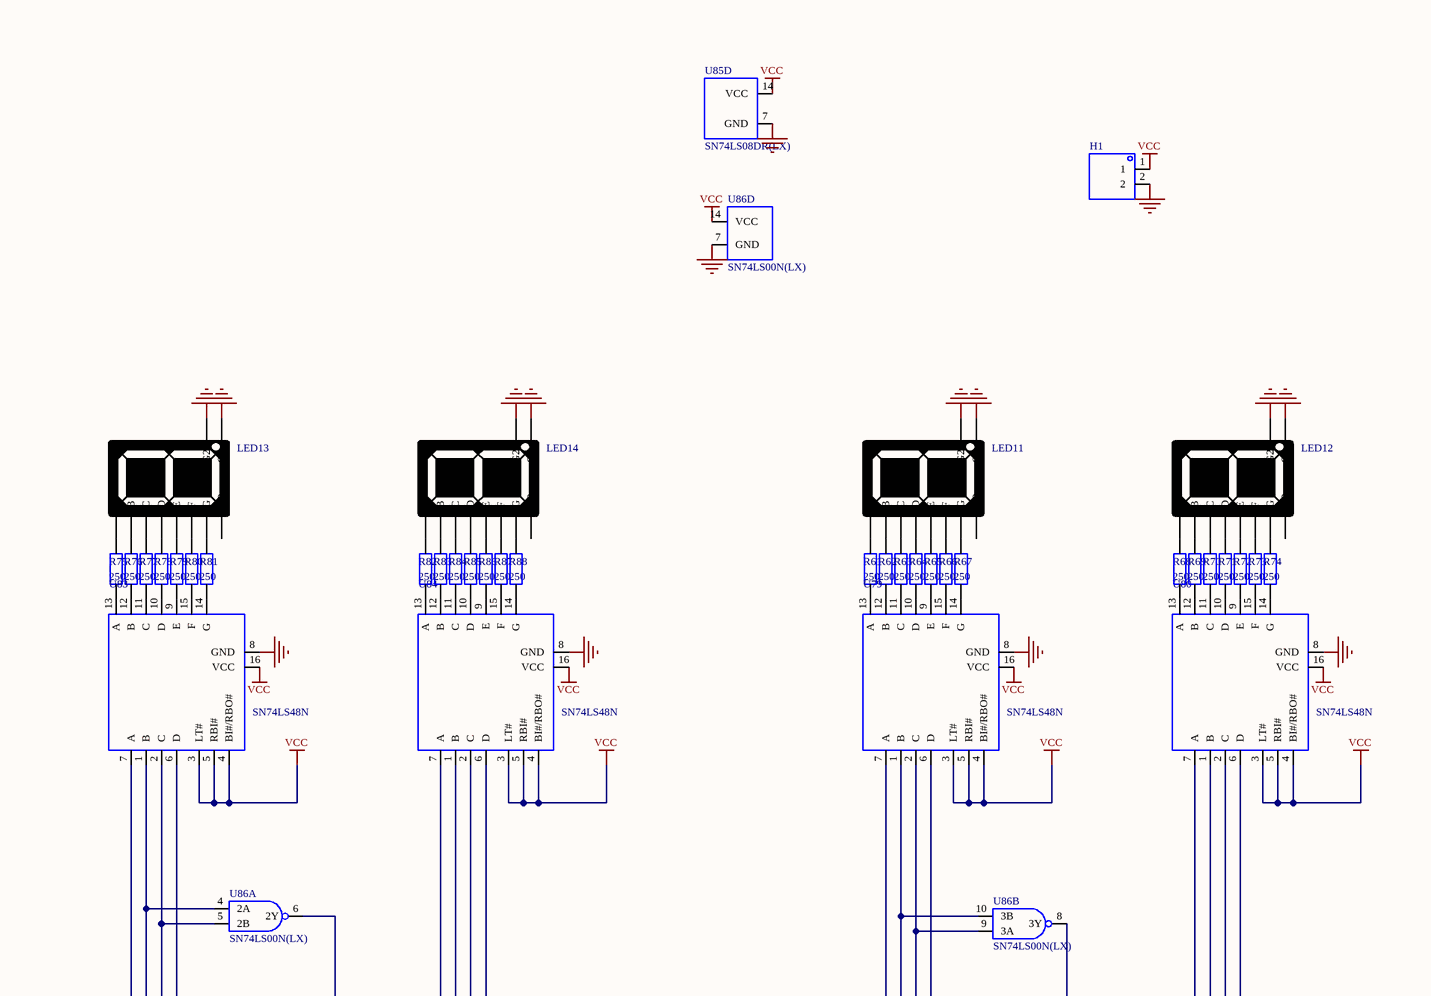
[diagram p0: MISC52151-3.schdoc, top left]
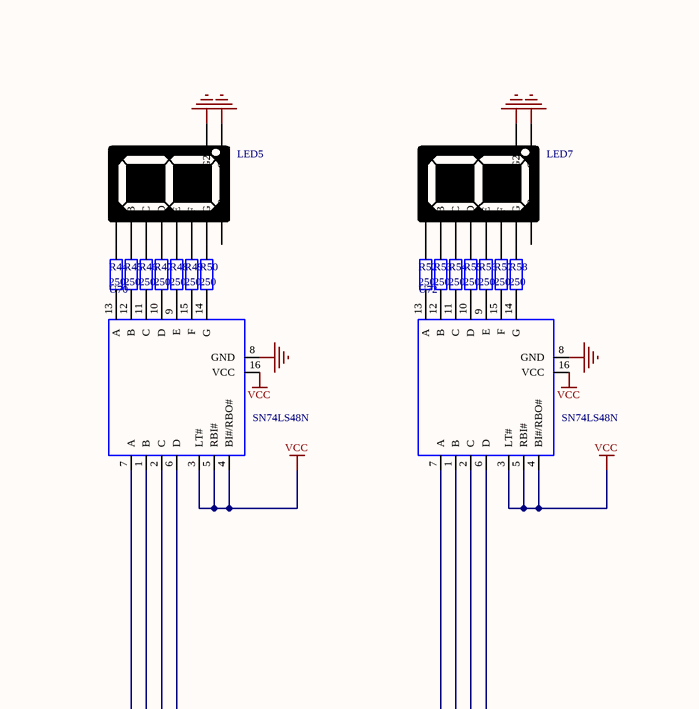
[diagram p1: MISC52151-3.schdoc, top right]
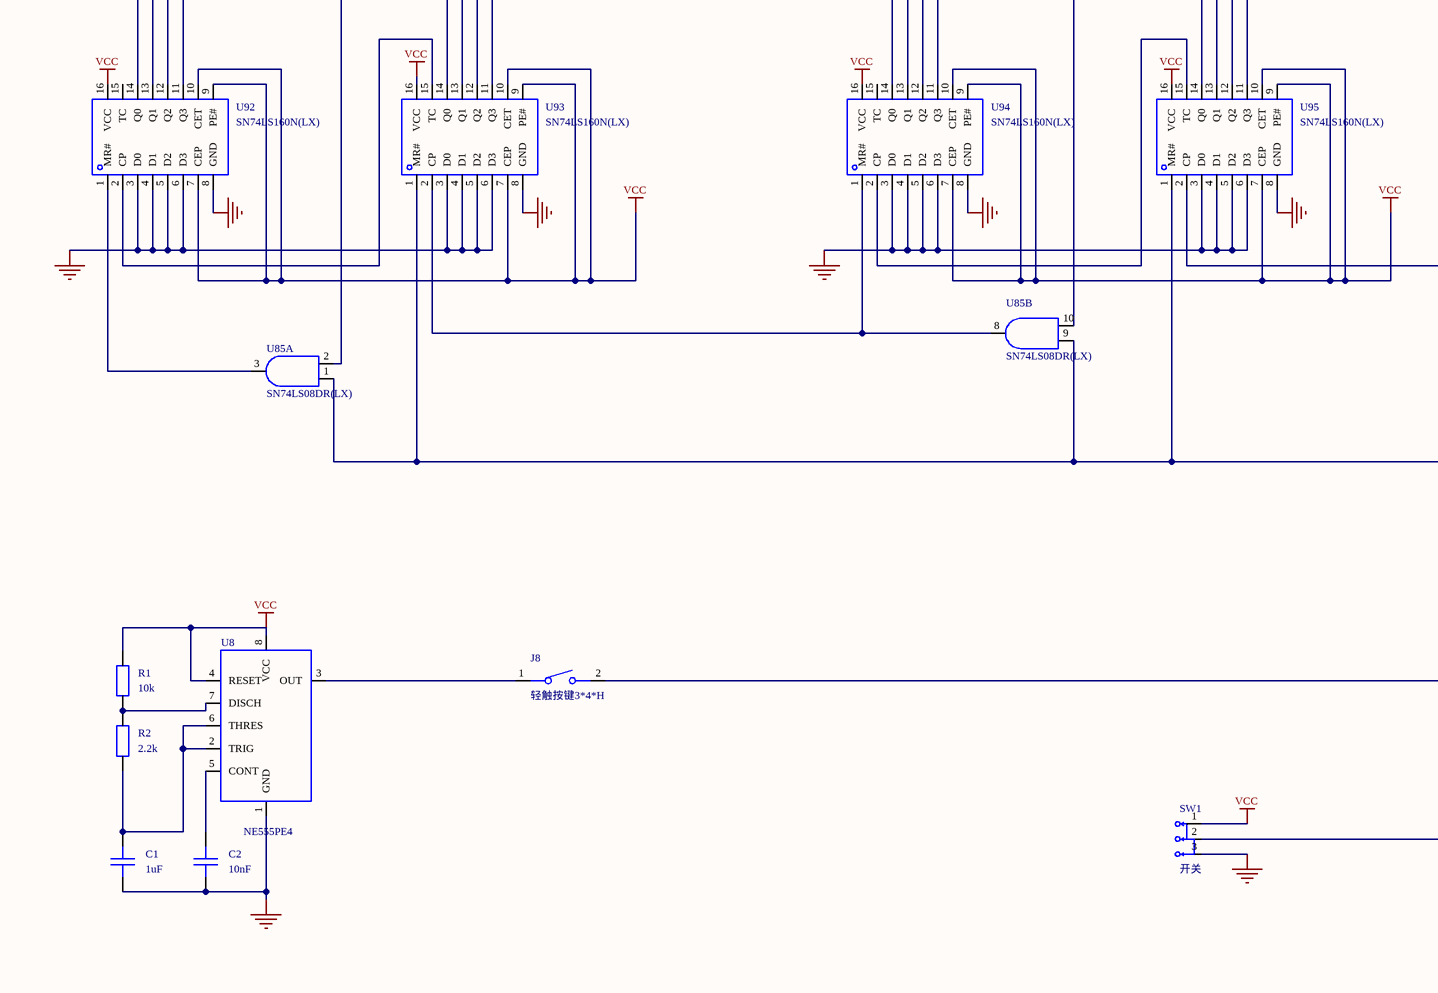
[diagram p2: MISC52151-3.schdoc, bottom left]
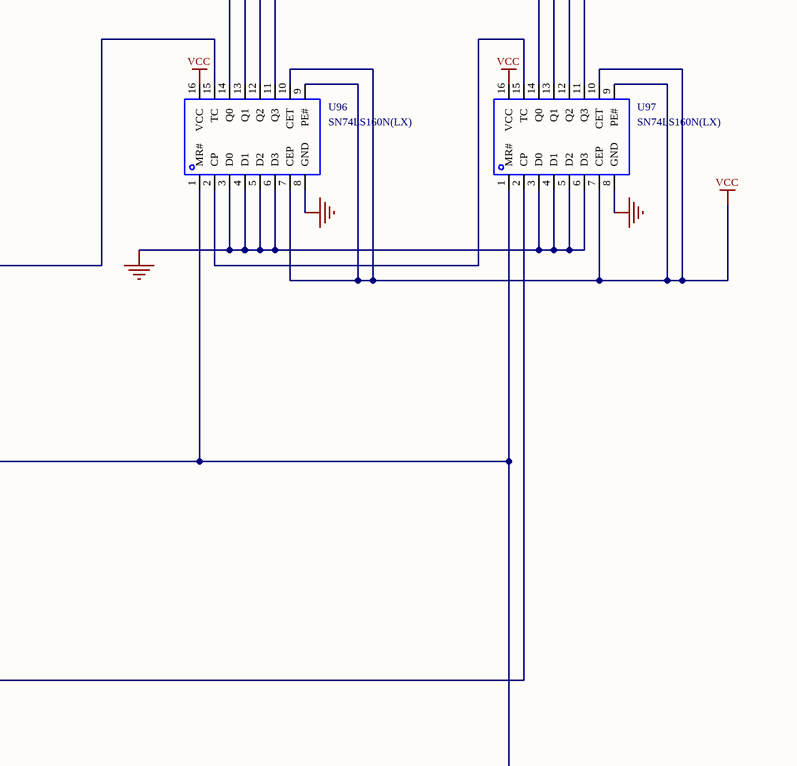
[diagram p3: MISC52151-3.schdoc, bottom right]
# Altium project MISC52151-2.PrjPcb
1 sheet, 70 parts. Net scope: global (net labels, ports and power ports of the same name join across sheets).
Board file: MISC52151.pcbdoc

## Sheet MISC52151-3.schdoc
size 178 x 98 mm; Version: V1.0; @Project Name: MISC52151; @Page Count: 1; @Update Date: 2025-06-06; @Create Date: 2025-06-06; @Schematic Name: MISC52151; @Page No: 1; @Board Name: MISC52151; @Create Time: 20:33:48; @Update Time: 02:46:09

### Parts
C1  1uF  [C0805]
C2  10nF  [C0805]
H1  (no value)  [HDR-TH_2P-P2.54-V-M-1]
J8  轻触按键3*4*H  [SW-SMD_L4.0-W2.9-LS5.0]
LED5  (no value)  [LED-SEG-TH_10P-L12.6-W19.0-P2.54-S15.24-BL]
LED7  (no value)  [LED-SEG-TH_10P-L12.6-W19.0-P2.54-S15.24-BL]
LED11  (no value)  [LED-SEG-TH_10P-L12.6-W19.0-P2.54-S15.24-BL]
LED12  (no value)  [LED-SEG-TH_10P-L12.6-W19.0-P2.54-S15.24-BL]
LED13  (no value)  [LED-SEG-TH_10P-L12.6-W19.0-P2.54-S15.24-BL]
LED14  (no value)  [LED-SEG-TH_10P-L12.6-W19.0-P2.54-S15.24-BL]
R1  10k  [R0603]
R2  2.2k  [R0603]
R44  250  [R0603]
R45  250  [R0603]
R46  250  [R0603]
R47  250  [R0603]
R48  250  [R0603]
R49  250  [R0603]
R50  250  [R0603]
R52  250  [R0603]
R53  250  [R0603]
R54  250  [R0603]
R55  250  [R0603]
R56  250  [R0603]
R57  250  [R0603]
R58  250  [R0603]
R61  250  [R0603]
R62  250  [R0603]
R63  250  [R0603]
R64  250  [R0603]
R65  250  [R0603]
R66  250  [R0603]
R67  250  [R0603]
R68  250  [R0603]
R69  250  [R0603]
R70  250  [R0603]
R71  250  [R0603]
R72  250  [R0603]
R73  250  [R0603]
R74  250  [R0603]
R75  250  [R0603]
R76  250  [R0603]
R77  250  [R0603]
R78  250  [R0603]
R79  250  [R0603]
R80  250  [R0603]
R81  250  [R0603]
R82  250  [R0603]
R83  250  [R0603]
R84  250  [R0603]
R85  250  [R0603]
R86  250  [R0603]
R87  250  [R0603]
R88  250  [R0603]
SW1  开关  [SW-TH_SS-12D01-GX]
U8  NE555PE4  [PDIP-8_L9.6-W6.4-P2.54-LS7.9-BL-1]
U70  SN74LS48N  [DIP-16_L19.3-W6.4-P2.54-LS7.6-BL]
U72  SN74LS48N  [DIP-16_L19.3-W6.4-P2.54-LS7.6-BL]
U79  SN74LS48N  [DIP-16_L19.3-W6.4-P2.54-LS7.6-BL]
U80  SN74LS48N  [DIP-16_L19.3-W6.4-P2.54-LS7.6-BL]
U83  SN74LS48N  [DIP-16_L19.3-W6.4-P2.54-LS7.6-BL]
U84  SN74LS48N  [DIP-16_L19.3-W6.4-P2.54-LS7.6-BL]
U85  SN74LS08DR(LX)  [SOIC-14_L8.7-W3.9-P1.27-LS6.0-BL]  (parts A,B,D of 4)
U86  SN74LS00N(LX)  [PDIP-14_L19.3-W6.4-P2.54-LS7.9-BL]  (parts A,B,D of 4)
U92  SN74LS160N(LX)  [DIP-16_L19.4-W6.4-P2.54-S7.6-BL]
U93  SN74LS160N(LX)  [DIP-16_L19.4-W6.4-P2.54-S7.6-BL]
U94  SN74LS160N(LX)  [DIP-16_L19.4-W6.4-P2.54-S7.6-BL]
U95  SN74LS160N(LX)  [DIP-16_L19.4-W6.4-P2.54-S7.6-BL]
U96  SN74LS160N(LX)  [DIP-16_L19.4-W6.4-P2.54-S7.6-BL]
U97  SN74LS160N(LX)  [DIP-16_L19.4-W6.4-P2.54-S7.6-BL]

### Nets
GND: C1.1 C2.1 H1.2 LED5.3(G1) LED5.8(G2) LED7.3(G1) LED7.8(G2) LED11.3(G1) LED11.8(G2) LED12.3(G1) LED12.8(G2) LED13.3(G1) LED13.8(G2) LED14.3(G1) LED14.8(G2) SW1.3 U8.1(GND) U70.8(GND) U72.8(GND) U79.8(GND) U80.8(GND) U83.8(GND) U84.8(GND) U85.7(GND) U86.7(GND) U92.3(D0) U92.4(D1) U92.5(D2) U92.6(D3) U92.8(GND) U93.3(D0) U93.4(D1) U93.5(D2) U93.6(D3) U93.8(GND) U94.3(D0) U94.4(D1) U94.5(D2) U94.6(D3) U94.8(GND) U95.3(D0) U95.4(D1) U95.5(D2) U95.6(D3) U95.8(GND) U96.3(D0) U96.4(D1) U96.5(D2) U96.6(D3) U96.8(GND) U97.3(D0) U97.4(D1) U97.5(D2) U97.6(D3) U97.8(GND)
VCC: H1.1 R1.2 SW1.1 U8.4(RESET) U8.8(VCC) U70.3(LT#) U70.4(BI#/RBO#) U70.5(RBI#) U70.16(VCC) U72.3(LT#) U72.4(BI#/RBO#) U72.5(RBI#) U72.16(VCC) U79.3(LT#) U79.4(BI#/RBO#) U79.5(RBI#) U79.16(VCC) U80.3(LT#) U80.4(BI#/RBO#) U80.5(RBI#) U80.16(VCC) U83.3(LT#) U83.4(BI#/RBO#) U83.5(RBI#) U83.16(VCC) U84.3(LT#) U84.4(BI#/RBO#) U84.5(RBI#) U84.16(VCC) U85.14(VCC) U86.14(VCC) U92.7(CEP) U92.9(PE#) U92.10(CET) U92.16(VCC) U93.7(CEP) U93.9(PE#) U93.10(CET) U93.16(VCC) U94.7(CEP) U94.9(PE#) U94.10(CET) U94.16(VCC) U95.7(CEP) U95.9(PE#) U95.10(CET) U95.16(VCC) U96.7(CEP) U96.9(PE#) U96.10(CET) U96.16(VCC) U97.7(CEP) U97.9(PE#) U97.10(CET) U97.16(VCC)
NetC1_2: C1.2 R2.1 U8.2(TRIG) U8.6(THRES)
NetC2_2: C2.2 U8.5(CONT)
NetJ8_1: J8.1 U8.3(OUT)
NetJ8_2: J8.2 U97.2(CP)
NetLED5_1: LED5.1(E) R48.2
NetLED5_2: LED5.2(D) R47.2
NetLED5_4: LED5.4(C) R46.2
NetLED5_6: LED5.6(B) R45.2
NetLED5_7: LED5.7(A) R44.2
NetLED5_9: LED5.9(F) R49.2
NetLED5_10: LED5.10(G) R50.2
NetLED7_1: LED7.1(E) R56.2
NetLED7_2: LED7.2(D) R55.2
NetLED7_4: LED7.4(C) R54.2
NetLED7_6: LED7.6(B) R53.2
NetLED7_7: LED7.7(A) R52.2
NetLED7_9: LED7.9(F) R57.2
NetLED7_10: LED7.10(G) R58.2
NetLED11_1: LED11.1(E) R65.2
NetLED11_2: LED11.2(D) R64.2
NetLED11_4: LED11.4(C) R63.2
NetLED11_6: LED11.6(B) R62.2
NetLED11_7: LED11.7(A) R61.2
NetLED11_9: LED11.9(F) R66.2
NetLED11_10: LED11.10(G) R67.2
NetLED12_1: LED12.1(E) R72.2
NetLED12_2: LED12.2(D) R71.2
NetLED12_4: LED12.4(C) R70.2
NetLED12_6: LED12.6(B) R69.2
NetLED12_7: LED12.7(A) R68.2
NetLED12_9: LED12.9(F) R73.2
NetLED12_10: LED12.10(G) R74.2
NetLED13_1: LED13.1(E) R79.2
NetLED13_2: LED13.2(D) R78.2
NetLED13_4: LED13.4(C) R77.2
NetLED13_6: LED13.6(B) R76.2
NetLED13_7: LED13.7(A) R75.2
NetLED13_9: LED13.9(F) R80.2
NetLED13_10: LED13.10(G) R81.2
NetLED14_1: LED14.1(E) R86.2
NetLED14_2: LED14.2(D) R85.2
NetLED14_4: LED14.4(C) R84.2
NetLED14_6: LED14.6(B) R83.2
NetLED14_7: LED14.7(A) R82.2
NetLED14_9: LED14.9(F) R87.2
NetLED14_10: LED14.10(G) R88.2
NetR1_1: R1.1 R2.2 U8.7(DISCH)
NetR44_1: R44.1 U70.13(A)
NetR45_1: R45.1 U70.12(B)
NetR46_1: R46.1 U70.11(C)
NetR47_1: R47.1 U70.10(D)
NetR48_1: R48.1 U70.9(E)
NetR49_1: R49.1 U70.15(F)
NetR50_1: R50.1 U70.14(G)
NetR52_1: R52.1 U72.13(A)
NetR53_1: R53.1 U72.12(B)
NetR54_1: R54.1 U72.11(C)
NetR55_1: R55.1 U72.10(D)
NetR56_1: R56.1 U72.9(E)
NetR57_1: R57.1 U72.15(F)
NetR58_1: R58.1 U72.14(G)
NetR61_1: R61.1 U79.13(A)
NetR62_1: R62.1 U79.12(B)
NetR63_1: R63.1 U79.11(C)
NetR64_1: R64.1 U79.10(D)
NetR65_1: R65.1 U79.9(E)
NetR66_1: R66.1 U79.15(F)
NetR67_1: R67.1 U79.14(G)
NetR68_1: R68.1 U80.13(A)
NetR69_1: R69.1 U80.12(B)
NetR70_1: R70.1 U80.11(C)
NetR71_1: R71.1 U80.10(D)
NetR72_1: R72.1 U80.9(E)
NetR73_1: R73.1 U80.15(F)
NetR74_1: R74.1 U80.14(G)
NetR75_1: R75.1 U83.13(A)
NetR76_1: R76.1 U83.12(B)
NetR77_1: R77.1 U83.11(C)
NetR78_1: R78.1 U83.10(D)
NetR79_1: R79.1 U83.9(E)
NetR80_1: R80.1 U83.15(F)
NetR81_1: R81.1 U83.14(G)
NetR82_1: R82.1 U84.13(A)
NetR83_1: R83.1 U84.12(B)
NetR84_1: R84.1 U84.11(C)
NetR85_1: R85.1 U84.10(D)
NetR86_1: R86.1 U84.9(E)
NetR87_1: R87.1 U84.15(F)
NetR88_1: R88.1 U84.14(G)
NetSW1_2: SW1.2 U85.1(1A) U85.9(3A) U93.1(MR#) U95.1(MR#) U96.1(MR#) U97.1(MR#)
NetU70_1: U70.1(B) U96.13(Q1)
NetU70_2: U70.2(C) U96.12(Q2)
NetU70_6: U70.6(D) U96.11(Q3)
NetU70_7: U70.7(A) U96.14(Q0)
NetU72_1: U72.1(B) U97.13(Q1)
NetU72_2: U72.2(C) U97.12(Q2)
NetU72_6: U72.6(D) U97.11(Q3)
NetU72_7: U72.7(A) U97.14(Q0)
NetU79_1: U79.1(B) U86.10(3B) U94.13(Q1)
NetU79_2: U79.2(C) U86.9(3A) U94.12(Q2)
NetU79_6: U79.6(D) U94.11(Q3)
NetU79_7: U79.7(A) U94.14(Q0)
NetU80_1: U80.1(B) U95.13(Q1)
NetU80_2: U80.2(C) U95.12(Q2)
NetU80_6: U80.6(D) U95.11(Q3)
NetU80_7: U80.7(A) U95.14(Q0)
NetU83_1: U83.1(B) U86.4(2A) U92.13(Q1)
NetU83_2: U83.2(C) U86.5(2B) U92.12(Q2)
NetU83_6: U83.6(D) U92.11(Q3)
NetU83_7: U83.7(A) U92.14(Q0)
NetU84_1: U84.1(B) U93.13(Q1)
NetU84_2: U84.2(C) U93.12(Q2)
NetU84_6: U84.6(D) U93.11(Q3)
NetU84_7: U84.7(A) U93.14(Q0)
NetU85_2: U85.2(1B) U86.6(2Y)
NetU85_3: U85.3(1Y) U92.1(MR#)
NetU85_8: U85.8(3Y) U93.2(CP) U94.1(MR#)
NetU85_10: U85.10(3B) U86.8(3Y)
NetU92_2: U92.2(CP) U93.15(TC)
NetU94_2: U94.2(CP) U95.15(TC)
NetU95_2: U95.2(CP) U96.15(TC)
NetU96_2: U96.2(CP) U97.15(TC)

Not connected (* = marked no-connect by the designer): LED5 5(DP); LED7 5(DP); LED11 5(DP); LED12 5(DP); LED13 5(DP); LED14 5(DP); U92 15(TC); U94 15(TC)

### Notes on the sheet
- 2025-06-06
- 原理图
- P1
- 版本
- 尺寸
- 页
- 共
- A4
- 1

### Library data of the parts
C1 C2 = CAP_0805: ConvertToPcb: yes; SymbolName: CapAcitance; ModelId: 1ba041120af144c991958decab20d241; ModelName: C0805_L2.0-W1.3-H1.3; ModelTransform: 78.74,51.181,0,0,0,0,0,0.0005,0; Device: CAP_0805; AddInBom: yes; Supplier Footprint: 0805; FootprintName: C0805
  C1: Value: 1uF
  C2: Value: 10nF
H1 = HDR-M_2.54_1x2P: Symbol: 210S-1*2P L=11.6MMGold-plated black; ConvertToPcb: yes; ModelId: 79b2e9f2d70a4d68a1b7098f27c6d4c5; ModelName: HDR-M-2.54_1x2; ModelTransform: 200,100,0,0,0,0,0,0,-118.11; Device: HDR-M_2.54_1x2P; AddInBom: yes; SupplierPart: C124375; Supplier Footprint: 插件; FootprintName: HDR-TH_2P-P2.54-V-M-1
J8 = 轻触按键3*4*H: AddInBom: yes; ModelId: 63599cce708d48afbce1b0db00354477; ModelName: SW-SMD_L4.0-W2.9-H2-LS5.0; ModelTransform: 196.85,114.173,0,0,0,0,0,0,0; Symbol: 轻触按键3*4*H; Device: 轻触按键3*4*H; LCSC Part Name: 轻触按键3*4*H; SupplierPart: C9900017573; ManufacturerPart: 轻触按键3*4*H; Supplier Footprint: 轻触按键3*4*2.5; Supplier: LCSC; ConvertToPcb: yes; FootprintName: SW-SMD_L4.0-W2.9-LS5.0
LED5 LED7 LED11-LED14 = LED_SEG_TH_0.56x1: Symbol: LED_SEG_TH_0.56*1; ConvertToPcb: yes; ModelId: 16c3aae6d39e4ecc9e744d6eeac8d57b; ModelName: LED-SEG-TH_0.56_1p; ModelTransform: 496.062,748.03,0,0,0,0,0,0,-137.795; Device: LED_SEG_TH_0.56x1; AddInBom: yes; Supplier Footprint: 插件; FootprintName: LED-SEG-TH_10P-L12.6-W19.0-P2.54-S15.24-BL
R1 R2 R44-R50 R52-R58 R61-R88 = Res_0603: Symbol: 电阻; ConvertToPcb: yes; ModelId: fc143cca1e79419f9cd78b61e9279f08; ModelTransform: 31.8897,63.7794,0,90,0,0,0,0,0; Device: Res_0603; AddInBom: yes; Supplier Footprint: 0603; FootprintName: R0603; ModelName: R0603
  R1: Value: 10k
  R2: Value: 2.2k
  R44-R50 R52-R58 R61-R88: Value: 250
SW1 = 开关: AddInBom: yes; ModelId: 46ec4e06866345239622c383c14b792d; ModelTransform: 346.456,153.543,0,0,0,0,-0.005,0,-169.291; Symbol: 开关; Device: 开关; LCSC Part Name: 开关; SupplierPart: C9900023015; ManufacturerPart: 开关; Supplier Footprint: SW-TH; Supplier: LCSC; ConvertToPcb: yes; FootprintName: SW-TH_SS-12D01-GX; ModelName: SW-TH_SS-12D01-GX
U8 = NE555PE4: 单精度计时器 8-PDIP 0 to 70; Manufacturer: TI(德州仪器); AddInBom: yes; ModelId: 1b8eaf096e7944deafe216467068c10e; ModelTransform: 377.952,318.897,0,0,0,0,0,0,-118.11; Symbol: NE555PE4; Device: NE555PE4; LCSC Part Name: NE555PE4; SupplierPart: C2859604; ManufacturerPart: NE555PE4; Supplier Footprint: PDIP-8; Datasheet: https://www.ti.com/cn/lit/gpn/sa555; Supplier: LCSC; ConvertToPcb: yes; FootprintName: PDIP-8_L9.6-W6.4-P2.54-LS7.9-BL-1; ModelName: PDIP-8_L9.6-W6.4-P2.54-LS7.9-BL-1
U70 U72 U79 U80 U83 U84 = SN74LS48N: Manufacturer: LX(灵星芯微); AddInBom: yes; ModelId: 6a0b9f170db542aa9e288f652469859c; ModelTransform: 759.841,309.842,0,0,0,0,0,0,-118.11; Symbol: SN74LS48N; Device: SN74LS48N; LCSC Part Name: SN74LS48N; SupplierPart: C22466304; ManufacturerPart: SN74LS48N; Supplier Footprint: DIP-16; JLCPCB Part Class: 扩展库; Datasheet: https://atta.szlcsc.com/upload/public/pdf/source/20240708/446E17B64DB311C394904D2DDEF6E8A1.pdf; Supplier: LCSC; ConvertToPcb: yes; FootprintName: DIP-16_L19.3-W6.4-P2.54-LS7.6-BL; ModelName: DIP-16_L19.3-W6.4-P2.54-LS7.6-BL
U85 = SN74LS08DR(LX): 逻辑类型:与门;通道数:4;电源电压:2V~6V;静态电流(最大值):2uA;最大传播延迟:15ns@6V;; Manufacturer: LX(灵星芯微); Relevance: []; AddInBom: yes; Logic Gate Type: 与门; Number of Channels: 4; Supply Voltage: 2V~6V; Quiescent Current (Max): 2uA; Sink Current: 5.2mA; High Level Range (VIH): 1.5V~4.2V; Low Level Range (VIL): 500mV~1.8V; ModelId: 8dbf5b715d42428c85558507ae5a252b; ModelName: SOIC-14_L8.6-W3.9-H1.8-LS6.0-P1.27; ModelTransform: 338.583,236.22,0,0,0,0,0,-0.001,0; Device: SN74LS08DR(LX); LCSC Part Name: 集成电路; SupplierPart: C22384802; ManufacturerPart: SN74LS08DR(LX); Supplier Footprint: SOP-14; Datasheet: https://atta.szlcsc.com/upload/public/pdf/source/20240417/39D5CB7746FCA2B194C58FD97B1F3E32.pdf; Supplier: LCSC; ConvertToPcb: yes; Source Current: 5.2mA; Series: 74LS系列; Propagation Delay Time: 15ns@6V; Operating Temperature: -40℃~+125℃; SymbolName: SN74LS08DR(LX); FootprintName: SOIC-14_L8.7-W3.9-P1.27-LS6.0-BL
U86 = SN74LS00N(LX): 逻辑类型:与非门;通道数:4;电源电压:2V~6V;静态电流(最大值):2uA;最大传播延迟:7ns@6V;; Manufacturer: LX(灵星芯微); Relevance: []; AddInBom: yes; Logic Gate Type: 与非门; Number of Channels: 4; Supply Voltage: 2V~6V; Quiescent Current (Max): 2uA; Sink Current: 5.2mA; High Level Range (VIH): 1.2V~3.2V; Low Level Range (VIL): 800mV~2.8V; Propagation Delay Time: 7ns@6V; ModelId: ed65e85d32ac41798f005e95ecc59a64; ModelTransform: 759.841,309.842,0,0,0,0,0,0,-118.11; Device: SN74LS00N(LX); LCSC Part Name: SN74LS00N(LX); SupplierPart: C22374089; ManufacturerPart: SN74LS00N(LX); Supplier Footprint: DIP-14; JLCPCB Part Class: 扩展库; Datasheet: https://atta.szlcsc.com/upload/public/pdf/source/20240402/5C5C61F6856D913ABEF0173ADDE42D20.pdf; Supplier: LCSC; ConvertToPcb: yes; Source Current: 5.2mA; Series: 74LS系列; Operating Temperature: -40℃~+125℃; SymbolName: SN74LS00N(LX); FootprintName: PDIP-14_L19.3-W6.4-P2.54-LS7.9-BL; ModelName: PDIP-14_L19.3-W6.4-P2.54-LS7.9-BL
U92-U97 = SN74LS160N(LX): 工作电压:2V~6V;触发沿:上升沿;计数速率:35MHz;; Manufacturer: LX(灵星芯微); AddInBom: yes; ModelId: c1b6497724fb4150b66e747391dddb83; ModelTransform: 763.77808,309.842,0,0,0,0,0,0,-129.921; Logic Type: 10分频; Voltage - Supply: 2V~6V; Trigger Type: 上升沿; Reset: 异步; Timing: 同步; Count Rate: 35MHz; Symbol: SN74LS160N(LX); Device: SN74LS160N(LX); LCSC Part Name: SN74LS160N(LX); SupplierPart: C22449620; ManufacturerPart: SN74LS160N(LX); Supplier Footprint: DIP-16; JLCPCB Part Class: 扩展库; Datasheet: https://atta.szlcsc.com/upload/public/pdf/source/20240603/B3BA67B8C0367C6F344464F1EF0FA571.pdf; Supplier: LCSC; ConvertToPcb: yes; FootprintName: DIP-16_L19.4-W6.4-P2.54-S7.6-BL; ModelName: DIP-16_L19.4-W6.4-P2.54-S7.6-BL; Operating Temperature: -40℃~+125℃